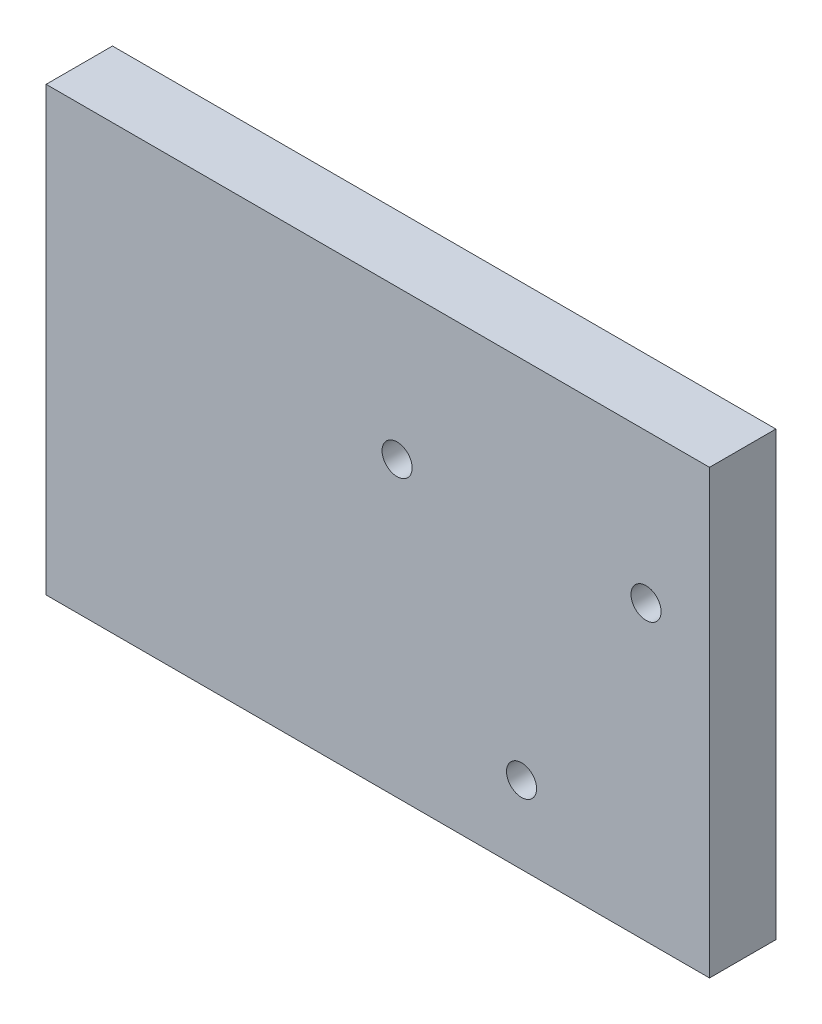
from build123d import *

# Parameters (mm, degrees)
SKETCH1_W             = 150
SKETCH1_H             = 100
BOSS_EXTRUDE1_DEPTH   = 15
M8_TAPPED_HOLE1_D     = 6.8
M8_TAPPED_HOLE1_DEPTH = 19.75
M8_TAPPED_HOLE1_TIP   = 2.042926105


with BuildPart() as part:
    # Sketch1 → Boss-Extrude1 (new body)
    with BuildSketch(Plane.XY):
        Rectangle(SKETCH1_W, SKETCH1_H)
    extrude(amount=BOSS_EXTRUDE1_DEPTH)

    # M8 Tapped Hole1
    with Locations(Plane.XY.offset(15)):
        with Locations((4.354174377, 16.25), (60.645825623, 16.25), (32.5, -32.5)):
            Hole(M8_TAPPED_HOLE1_D / 2, depth=M8_TAPPED_HOLE1_DEPTH)
            with Locations((0, 0, -(M8_TAPPED_HOLE1_DEPTH + M8_TAPPED_HOLE1_TIP / 2))):  # 118° drill point
                Cone(0, M8_TAPPED_HOLE1_D / 2, M8_TAPPED_HOLE1_TIP, mode=Mode.SUBTRACT)


solid = part.part
